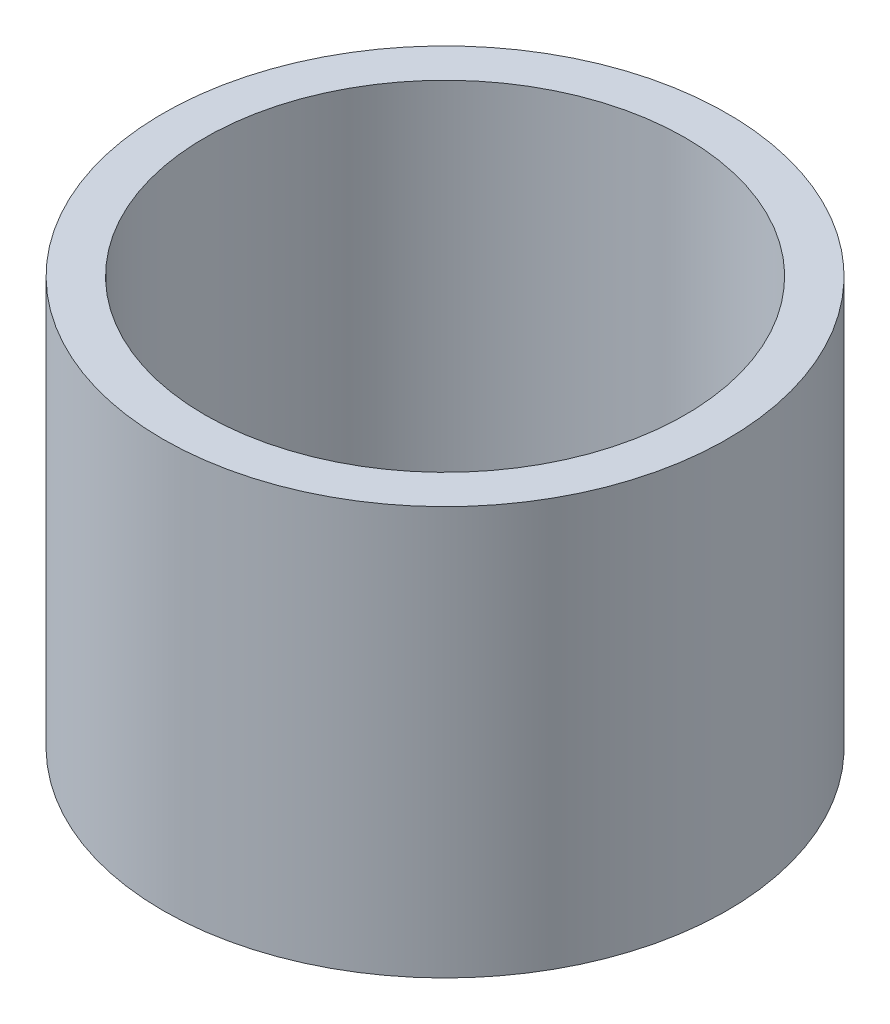
SolidWorks part; units mm, degrees
ref_plane "前视基准面" through (0, 0, 0) normal (0, 0, 1) x (1, 0, 0)
ref_plane "上视基准面" through (0, 0, 0) normal (0, 1, 0) x (1, 0, 0)
ref_plane "右视基准面" through (0, 0, 0) normal (1, 0, 0) x (0, 0, -1)
sketch "草图1" plane through (0, 0, 0) normal (0, 1, 0) x (1, 0, 0)
  circle A0 centre (0, 0) radius 23.5
  circle A1 centre (0, 0) radius 20
  dimension "D1" = 47
  dimension "D2" = 40
extrude "凸台-拉伸1" add sketch "草图1" along normal blind 34
